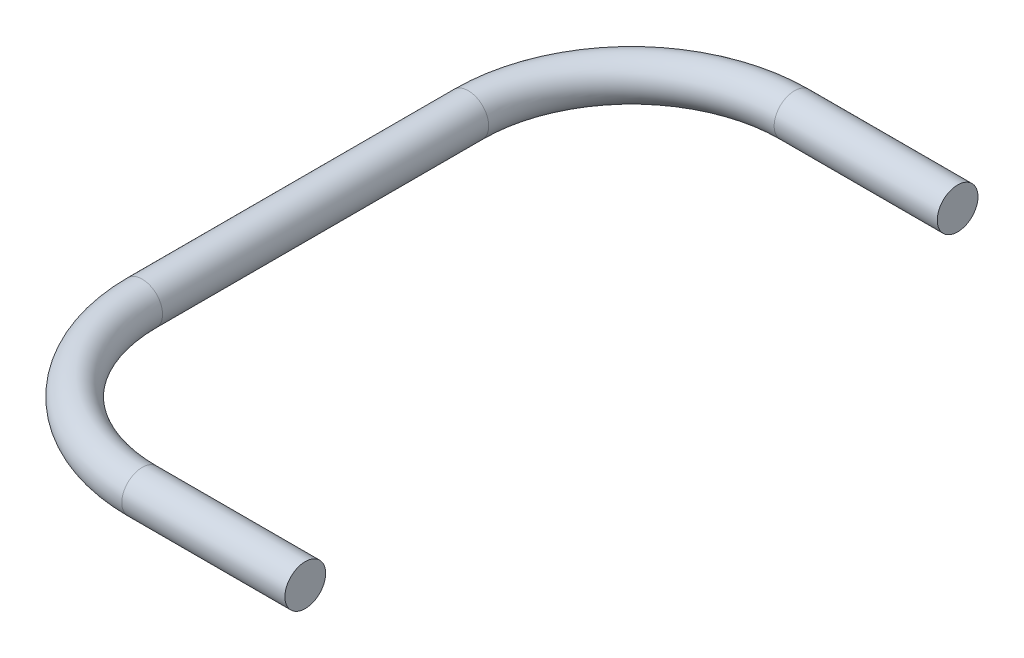
SolidWorks part; units mm, degrees
ref_plane "Front Plane" through (0, 0, 0) normal (0, 0, 1) x (1, 0, 0)
ref_plane "Top Plane" through (0, 0, 0) normal (0, 1, 0) x (1, 0, 0)
ref_plane "Right Plane" through (0, 0, 0) normal (1, 0, 0) x (0, 0, -1)
sketch "Sketch1" plane through (0, 0, 0) normal (0, 1, 0) x (1, 0, 0)
  line L0 (0, 0) -> (-20, 0)
  line L1 (-40, -20) -> (-40, -60)
  line L2 (-20, -80) -> (0, -80)
  arc A0 (-20, 0) -> (-40, -20) centre (-20, -20) ccw
  arc A1 (-20, -80) -> (-40, -60) centre (-20, -60) cw
  point P7 (-40, 0)
  point P10 (-40, -80)
  dimension "D3" = 20
  dimension "D4" = 20
  dimension "D1" = 40
  dimension "D2" = 80
sketch "Sketch2" plane through (0, 0, 0) normal (1, 0, 0) x (0, 0, -1)
  circle A0 centre (0, 0) radius 2.5
  dimension "D1" = 5
sweep "Sweep1" add profiles "Sketch2" path "Sketch1"
